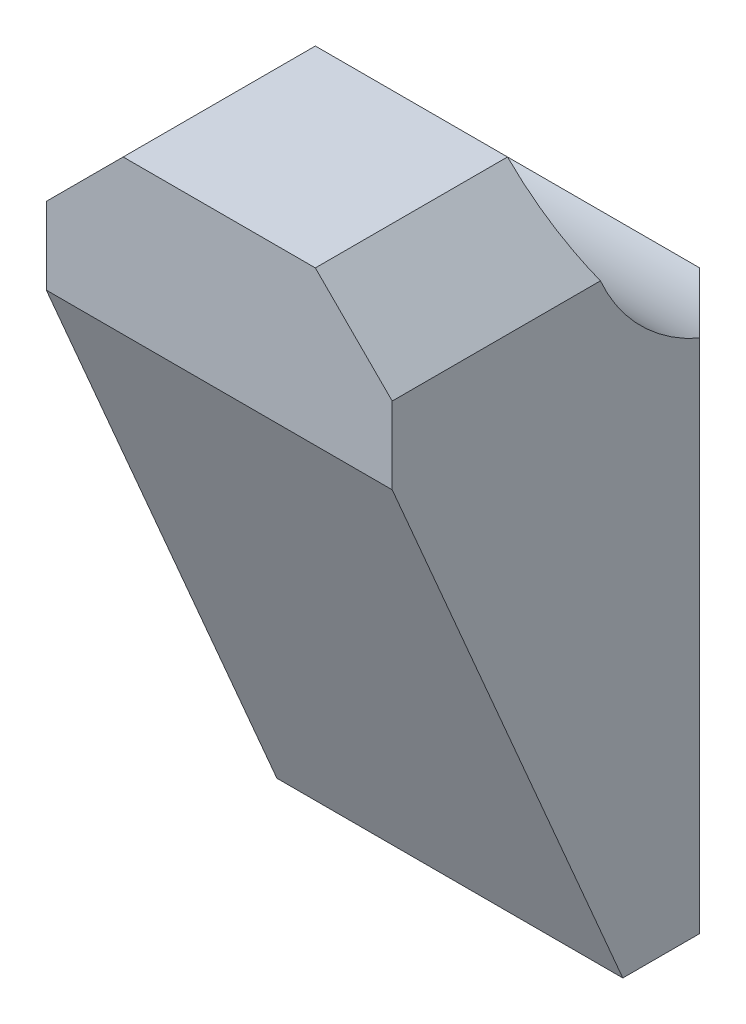
from build123d import *

# Parameters (mm, degrees)
BOSS_EXTRUDE1_DEPTH = 22.5
CHAMFER1_SIZE       = 10


with BuildPart() as part:
    # Sketch1 → Boss-Extrude1 (new, symmetric)
    with BuildSketch(Plane(origin=(0, 0, 0), x_dir=(0, 0, -1), z_dir=(1, 0, 0))):
        with BuildLine():
            Line((0, 0), (0, 65))
            ThreePointArc((0, 65), (-17.67766953, 72.32233047), (-25, 90))
            Line((-25, 90), (-50, 90))
            Line((-50, 90), (-50, 70))
            Line((-50, 70), (-20, 0))
            Line((-20, 0), (0, 0))
        make_face()
    extrude(amount=BOSS_EXTRUDE1_DEPTH, both=True)

    # Chamfer1
    chamfer1_edges = [part.edges().sort_by_distance(p)[0] for p in [
        (22.5, 90, 37.5),
        (-22.5, 90, 37.5),
        (22.5, 32.5, 0),
        (-22.5, 32.5, 0),
    ]]
    chamfer(chamfer1_edges, length=CHAMFER1_SIZE)


solid = part.part
